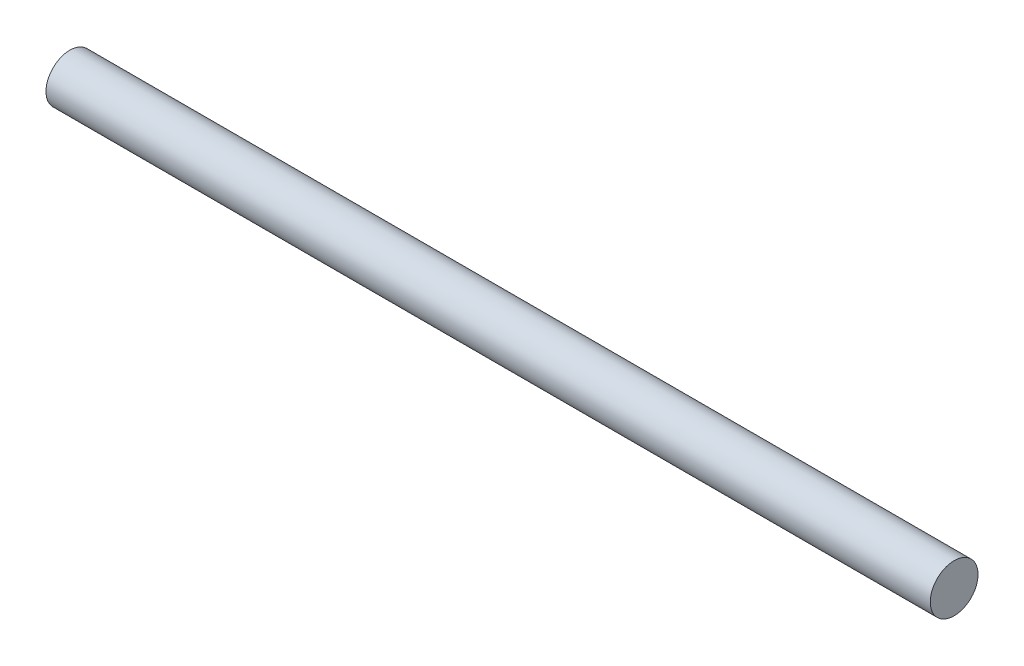
SolidWorks part; units mm, degrees
material "普通碳钢"
ref_plane "Front Plane" through (0, 0, 0) normal (0, 0, 1) x (1, 0, 0)
ref_plane "Top Plane" through (0, 0, 0) normal (0, 1, 0) x (1, 0, 0)
ref_plane "Right Plane" through (0, 0, 0) normal (1, 0, 0) x (0, 0, -1)
sketch "Sketch1" plane through (0, 0, 0) normal (0, 0, 1) x (1, 0, 0)
  line L0 (-202.6045, 0) -> (262.3615, 0) construction
  line L1 (-185, 0) -> (-185, 10)
  line L2 (-185, 10) -> (0, 10)
  line L3 (0, 10) -> (0, 0)
  line L6 (0, 0) -> (-185, 0)
  dimension "D1" = 185
  dimension "D4" = 10
revolve "Revolve1" add sketch "Sketch1" angle 360 about L0
sketch "Sketch3" plane through (-185, 0, 0) normal (-1, 0, 0) x (0, 0, 1)
  line L2 (-8.5, 5.2678) -> (-8.5, -5.2678)
  line L4 (8.5, 5.2678) -> (8.5, -5.2678)
  arc A0 (-8.5, 5.2678) -> (-8.5, -5.2678) centre (0, 0) ccw
  circle A1 centre (0, 0) radius 10
  arc A2 (8.5, -5.2678) -> (8.5, 5.2678) centre (0, 0) ccw
  dimension "D2" = 17
  dimension "D3" = 8.5
  dimension "D1" = 0
extrude "Cut-Extrude1" [suppressed] cut sketch "Sketch3" against normal blind 17
mirror "Mirror1" about plane through (0, 0, 0) normal (1, 0, 0) of "Cut-Extrude1", "Revolve1"
